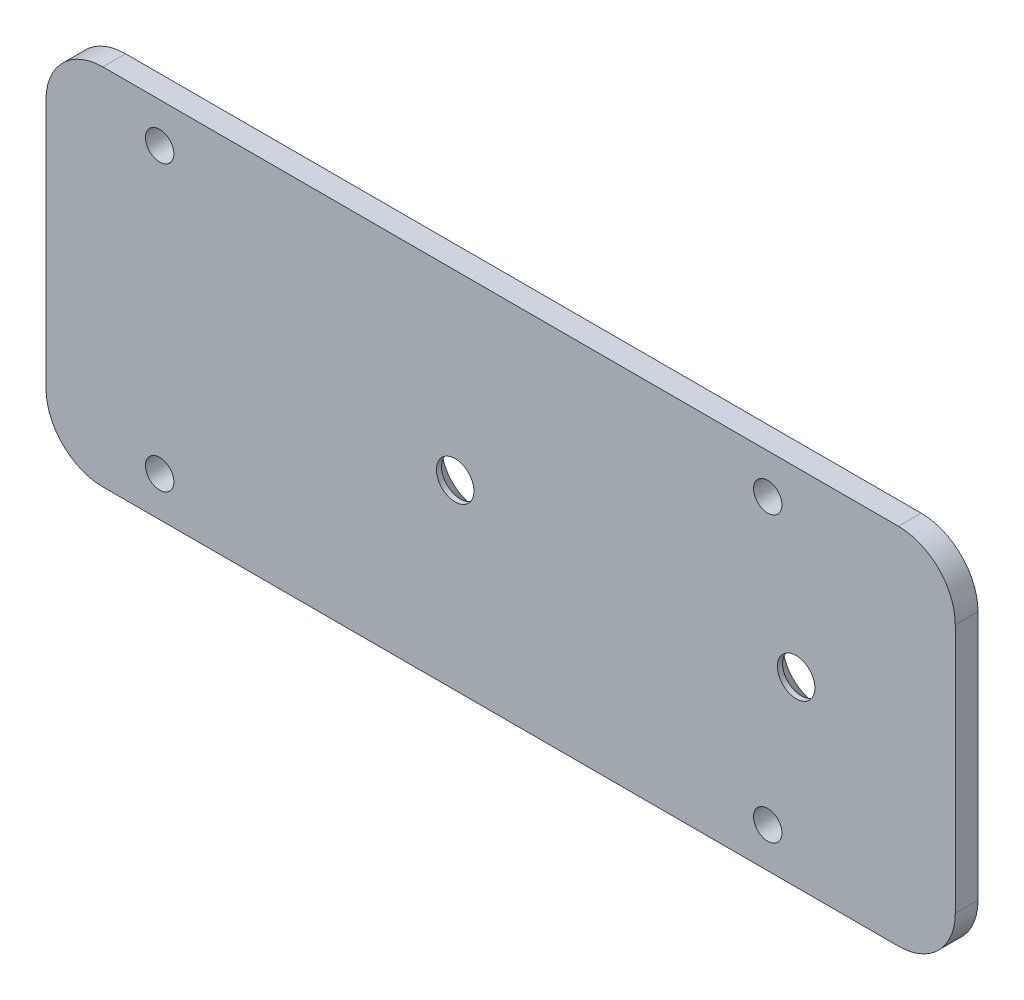
SolidWorks part; units mm, degrees
material "6061 GB/T6892-2006"
ref_plane "前视基准面" through (0, 0, 0) normal (0, 0, 1) x (1, 0, 0)
ref_plane "上视基准面" through (0, 0, 0) normal (0, 1, 0) x (1, 0, 0)
ref_plane "右视基准面" through (0, 0, 0) normal (1, 0, 0) x (0, 0, -1)
sketch "草图1" plane through (0, 0, 0) normal (0, 0, 1) x (1, 0, 0)
  line L5 (-80, 32) -> (80, 32)
  line L6 (-80, 32) -> (-80, -32)
  line L7 (-80, -32) -> (80, -32)
  line L8 (80, 32) -> (80, -32)
  line L9 (-80, 32) -> (80, -32) construction
  line L10 (-80, -32) -> (80, 32) construction
  point P0 (0, 0)
  dimension "D1" = 64
  dimension "D2" = 160
extrude "凸台-拉伸1" add sketch "草图1" along normal blind 4
fillet "圆角1" radius 10 4 edges at (80, 32, 2) (80, -32, 2) (-80, 32, 2) (-80, -32, 2)
hole_wizard "M6 螺纹孔1" positions "草图3" profile "草图4" tap size "M6" standard "GB" end condition through all
sketch "草图3" plane through (0, 0, 4) normal (0, 0, 1) x (1, 0, 0)
  line L0 (-80, 22) -> (-80, -22) construction
  line L3 (0, 0) -> (48.6927, 0) construction
  point P0 (-60, 25)
  point P2 (-60, -25)
  point P4 (47, 25)
  point P6 (47, -25)
  dimension "D1" = 20
  dimension "D2" = 50
  dimension "D3" = 20
  dimension "D4" = 107
sketch "草图4" plane through (-60, 25, 4) normal (1, 0, 0) x (0, -1, 0)
  line L0 (0, 0) -> (0, 4)
  line L1 (0, 4) -> (2.5, 4)
  line L2 (2.5, 4) -> (2.5, 0)
  line L5 (2.5, 0) -> (0, 0)
  line L11 (0, -6.35) -> (0, 107.95) construction
  dimension "通孔螺纹孔钻头直径" = 5
  dimension "通孔螺纹孔钻头深度" = 4
cosmetic thread "孔螺蚊线1"
cosmetic thread "孔螺蚊线2"
cosmetic thread "孔螺蚊线3"
cosmetic thread "孔螺蚊线4"
hole_wizard "打孔尺寸(%根据)内六角花形半沉头螺钉的类型2" positions "草图5" profile "草图6" countersink size "M6" standard "GB" end condition through all
sketch "草图5" plane through (0, 0, 0) normal (0, 0, -1) x (-1, 0, 0)
  line L0 (80, 22) -> (80, -22) construction
  point P0 (-52, 0)
  point P2 (8, 0)
  dimension "D1" = 72
  dimension "D2" = 60
sketch "草图6" plane through (52, 0, 0) normal (1, 0, 0) x (0, 1, 0)
  line L0 (0, 0) -> (0, 4)
  line L1 (0, 4) -> (3.3, 4)
  line L2 (3.3, 4) -> (3.3, 3.1)
  line L3 (3.3, 3.1) -> (6.4, 0)
  line L5 (6.4, 0) -> (0, 0)
  line L6 (-3.3, 3.1) -> (-6.4, 0) construction
  line L11 (0, -6.35) -> (0, 107.95) construction
  dimension "通孔孔直径" = 6.6
  dimension "通孔孔深度" = 4
  dimension "近端锥形沉头孔直径" = 12.8
  dimension "近端锥形沉头孔角度" = 90
